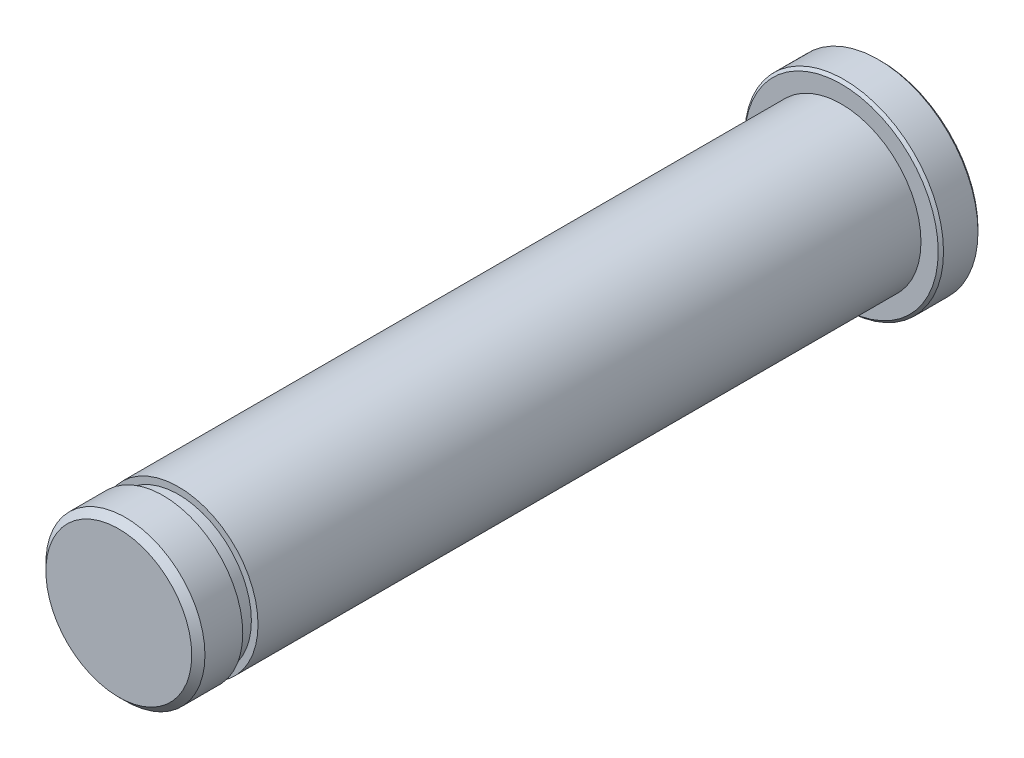
SolidWorks part; units mm, degrees
ref_plane "Front Plane" through (0, 0, 0) normal (0, 0, 1) x (1, 0, 0)
ref_plane "Top Plane" through (0, 0, 0) normal (0, 1, 0) x (1, 0, 0)
ref_plane "Right Plane" through (0, 0, 0) normal (1, 0, 0) x (0, 0, -1)
sketch "Sketch1" plane through (0, 0, 0) normal (0, 0, 1) x (1, 0, 0)
  circle A0 centre (0, 0) radius 7.5
  dimension "D1" = 15
extrude "Boss-Extrude1" add sketch "Sketch1" along normal blind 3
sketch "Sketch2" plane through (0, 0, 3) normal (0, 0, 1) x (1, 0, 0)
  circle A0 centre (0, 0) radius 6
  dimension "D1" = 12
extrude "Boss-Extrude2" add sketch "Sketch2" along normal blind 54.5
chamfer "Chamfer1" distance 0.2 angle 45 2 edges at (7.5, 0, 0) (7.5, 0, 3)
sketch "Sketch3" plane through (0, 0, 0) normal (0, 1, 0) x (1, 0, 0)
  line L0 (-6, -3) -> (-6, -57.5) construction
  line L1 (-6, -54.15) -> (-5.5, -54.15)
  line L2 (-6, -54.15) -> (-6, -53)
  line L3 (-6, -53) -> (-5.5, -53)
  line L4 (-5.5, -54.15) -> (-5.5, -53)
  line L5 (-6, -57.5) -> (6, -57.5) construction
  dimension "D1" = 0.5
  dimension "D2" = 1.15
  dimension "D3" = 3.35
ref_axis "Axis1" through (0, 0, 57.5) along (0, 0, -1)
revolve "Cut-Revolve1" cut sketch "Sketch3" angle 360 about axis through (0, 0, 57.5) along (0, 0, -1)
chamfer "Chamfer2" distance 0.5 angle 45 1 edges at (6, 0, 57.5)
